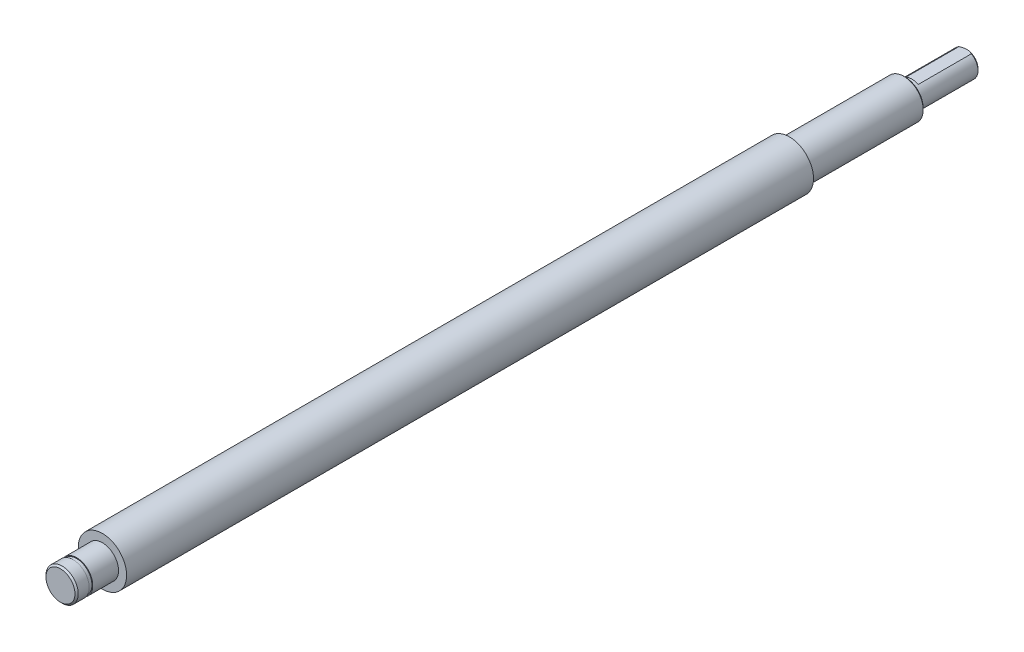
SolidWorks part; units mm, degrees
material "45钢"
ref_plane "前视基准面" through (0, 0, 0) normal (0, 0, 1) x (1, 0, 0)
ref_plane "上视基准面" through (0, 0, 0) normal (0, 1, 0) x (1, 0, 0)
ref_plane "右视基准面" through (0, 0, 0) normal (1, 0, 0) x (0, 0, -1)
sketch "草图1" plane through (0, 0, 0) normal (0, 0, 1) x (1, 0, 0)
  circle A0 centre (0, 0) radius 7.5
  dimension "D1" = 15
extrude "凸台-拉伸1" add sketch "草图1" along normal blind 281
sketch "草图3" plane through (0, 0, 0) normal (0, 1, 0) x (1, 0, 0)
  line L0 (0, -281) -> (0, 0) construction
  line L8 (-53.8738, -268) -> (-5, -268)
  line L9 (-53.8738, -268) -> (-53.8738, -281)
  line L10 (-53.8738, -281) -> (-5, -281)
  line L11 (-5, -268) -> (-5, -281)
  line L12 (-53.8738, -268) -> (-5, -281) construction
  line L13 (-53.8738, -281) -> (-5, -268) construction
  line L14 (-7.5, -281) -> (7.5, -281) construction
  point P8 (-29.4369, -274.5)
  dimension "D1" = 5
  dimension "D2" = 13
revolve "切除-旋转1" cut sketch "草图3" angle 360 about axis through (0, 0, 281) along (0, 0, -1)
sketch "草图4" plane through (0, 0, 0) normal (0, 1, 0) x (1, 0, 0)
  line L0 (0, -268) -> (0, 0) construction
  line L1 (41.8364, 27.6806) -> (6, 27.6806)
  line L2 (41.8364, 27.6806) -> (41.8364, -55)
  line L3 (41.8364, -55) -> (6, -55)
  line L4 (6, 27.6806) -> (6, -55)
  line L5 (41.8364, 27.6806) -> (6, -55) construction
  line L6 (41.8364, -55) -> (6, 27.6806) construction
  line L7 (7.5, 0) -> (-7.5, 0) construction
  point P0 (23.9182, -13.6597)
  dimension "D1" = 6
  dimension "D2" = 55
revolve "切除-旋转2" cut sketch "草图4" angle 360 about axis through (0, 0, 281) along (0, 0, -1)
cosmetic thread "装饰螺纹线1" parameters "D1"=30, "D2"=11
sketch "草图8" plane through (0, 0, 0) normal (0, 1, 0) x (1, 0, 0)
  line L0 (0, 0) -> (0, -55) construction
  line L1 (-37.1488, 20.7536) -> (-4, 20.7536)
  line L2 (-37.1488, 20.7536) -> (-37.1488, -19)
  line L3 (-37.1488, -19) -> (-4, -19)
  line L4 (-4, 20.7536) -> (-4, -19)
  line L5 (-37.1488, 20.7536) -> (-4, -19) construction
  line L6 (-37.1488, -19) -> (-4, 20.7536) construction
  line L8 (7.5, -55) -> (-7.5, -55) construction
  point P0 (-20.5744, 0.8768)
  dimension "D1" = 4
  dimension "D2" = 36
revolve "切除-旋转5" cut sketch "草图8" angle 360 about axis through (0, 0, 268) along (0, 0, 1)
ref_plane "基准面1" through (0, 5, 0) normal (0, 1, 0) x (1, 0, 0)
chamfer "倒角2" distance 0.5 angle 45 2 edges at (4, 0, 0) (6, 0, 19)
sketch "草图15" plane through (0, 0, 0) normal (0, 1, 0) x (1, 0, 0)
  line L0 (-5, -268) -> (5, -268) construction
  line L1 (-20.0409, -276) -> (-4.75, -276)
  line L2 (-20.0409, -276) -> (-20.0409, -277.1)
  line L3 (-20.0409, -277.1) -> (-4.75, -277.1)
  line L4 (-4.75, -276) -> (-4.75, -277.1)
  line L5 (-20.0409, -276) -> (-4.75, -277.1) construction
  line L6 (-20.0409, -277.1) -> (-4.75, -276) construction
  line L7 (-5, -268) -> (-5, -281) construction
  point P0 (-12.3954, -276.55)
  dimension "D1" = 8
  dimension "D2" = 0.25
  dimension "D3" = 1.1
revolve "切除-旋转7" cut sketch "草图15" angle 360 about axis through (0, 0, 281) along (0, 0, 1)
chamfer "倒角3" distance 0.5 angle 45 1 edges at (5, 0, 281)
sketch "草图16" plane through (0, 0, 0) normal (0, 0, -1) x (-1, 0, 0)
  line L1 (-18.031, 18.359) -> (9.0409, 18.359)
  line L2 (-18.031, 18.359) -> (-18.031, 3.5)
  line L3 (-18.031, 3.5) -> (9.0409, 3.5)
  line L4 (9.0409, 18.359) -> (9.0409, 3.5)
  line L5 (-18.031, 18.359) -> (9.0409, 3.5) construction
  line L6 (-18.031, 3.5) -> (9.0409, 18.359) construction
  point P0 (-4.495, 10.9295)
  dimension "D1" = 3.5
extrude "切除-拉伸1" cut sketch "草图16" against normal blind 17
